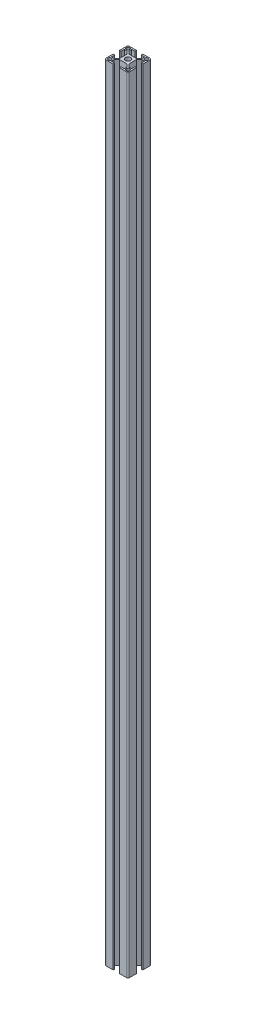
SolidWorks part; units mm, degrees
ref_plane "前视基准面" through (0, 0, 0) normal (0, 0, 1) x (1, 0, 0)
ref_plane "上视基准面" through (0, 0, 0) normal (0, 1, 0) x (1, 0, 0)
ref_plane "右视基准面" through (0, 0, 0) normal (1, 0, 0) x (0, 0, -1)
sketch "草图1" plane through (0, 0, 0) normal (0, 1, 0) x (1, 0, 0)
  line L44 (6.75, -28) -> (11, -28)
  line L45 (11, -28) -> (11, -30)
  line L46 (11, -30) -> (2, -30)
  line L47 (0, -28) -> (0, -19)
  line L48 (0, -19) -> (2, -19)
  line L49 (2, -19) -> (2, -23.25)
  line L50 (28, -30) -> (19, -30)
  line L51 (19, -30) -> (19, -28)
  line L52 (23.25, -28) -> (23.25, -24.6642)
  line L53 (19, -28) -> (23.25, -28)
  line L54 (30, -19) -> (30, -28)
  line L55 (28, -19) -> (30, -19)
  line L56 (28, -23.25) -> (28, -19)
  line L57 (24.6642, -23.25) -> (28, -23.25)
  line L58 (21, -19.5858) -> (24.6642, -23.25)
  line L59 (23.25, -24.6642) -> (19.5858, -21)
  line L60 (6.75, -24.6642) -> (6.75, -28)
  line L61 (2, -23.25) -> (5.3358, -23.25)
  line L62 (5.3358, -23.25) -> (9, -19.5858)
  line L63 (10.4142, -21) -> (6.75, -24.6642)
  line L64 (19.5858, -21) -> (10.4142, -21)
  line L65 (9, -19.5858) -> (9, -10.4142)
  line L66 (21, -10.4142) -> (21, -19.5858)
  line L67 (30, -11) -> (28, -11)
  line L68 (28, -11) -> (28, -6.75)
  line L69 (28, -6.75) -> (24.6642, -6.75)
  line L70 (24.6642, -6.75) -> (21, -10.4142)
  line L71 (19.5858, -9) -> (23.25, -5.3358)
  line L72 (10.4142, -9) -> (19.5858, -9)
  line L73 (6.75, -5.3358) -> (10.4142, -9)
  line L74 (9, -10.4142) -> (5.3358, -6.75)
  line L75 (2, -11) -> (0, -11)
  line L76 (2, -6.75) -> (2, -11)
  line L77 (5.3358, -6.75) -> (2, -6.75)
  line L78 (6.75, -2) -> (6.75, -5.3358)
  line L79 (23.25, -5.3358) -> (23.25, -2)
  line L80 (23.25, -2) -> (19, -2)
  line L81 (19, -2) -> (19, 0)
  line L82 (11, 0) -> (11, -2)
  line L83 (11, -2) -> (6.75, -2)
  line L84 (30, -2) -> (30, -11)
  line L85 (19, 0) -> (28, 0)
  line L86 (2, 0) -> (11, 0)
  line L87 (0, -11) -> (0, -2)
  line L88 (0, -15) -> (30, -15) construction
  line L89 (15, -30) -> (15, 0) construction
  line L90 (0, 0) -> (30, -30) construction
  line L91 (0, -30) -> (30, 0) construction
  arc A9 (0, -28) -> (2, -30) centre (2, -28) ccw
  circle A10 centre (3.375, -26.625) radius 2.1
  circle A11 centre (26.625, -26.625) radius 2.1
  arc A12 (28, -30) -> (30, -28) centre (28, -28) ccw
  circle A13 centre (15, -15) radius 3.4
  circle A14 centre (3.375, -3.375) radius 2.1
  circle A15 centre (26.625, -3.375) radius 2.1
  arc A16 (30, -2) -> (28, 0) centre (28, -2) ccw
  arc A17 (2, 0) -> (0, -2) centre (2, -2) ccw
  dimension "D2" = 15
  dimension "D5" = 6.8
  dimension "D8" = 6
  dimension "D11" = 23.25
  dimension "D12" = 3.375
  dimension "D13" = 23.25
  dimension "D14" = 4.2
  dimension "D15" = 2
  dimension "D16" = 2
  dimension "D23" = 2
  dimension "D24" = 2
  dimension "D1" = 15
  dimension "D3" = 45
  dimension "D4" = 45
  dimension "D6" = 30
  dimension "D7" = 30
  dimension "D9" = 12
  dimension "D10" = 3.375
  dimension "D17" = 11
  dimension "D18" = 8
  dimension "D19" = 2
  dimension "D20" = 2
  dimension "D21" = 11
  dimension "D22" = 8
  dimension "D25" = 2
  dimension "D26" = 2
  dimension "D27" = 6.75
  dimension "D28" = 16.5
  dimension "D29" = 6.75
  dimension "D30" = 16.5
  dimension "D31" = 12
  dimension "D32" = 6
  dimension "D33" = 2
  dimension "D34" = 1
  dimension "D35" = 2
  dimension "D36" = 1
extrude "拉伸1" add sketch "草图1" along normal blind 1000
cosmetic thread "装饰螺纹线1" parameters "D1"=15, "D2"=8
